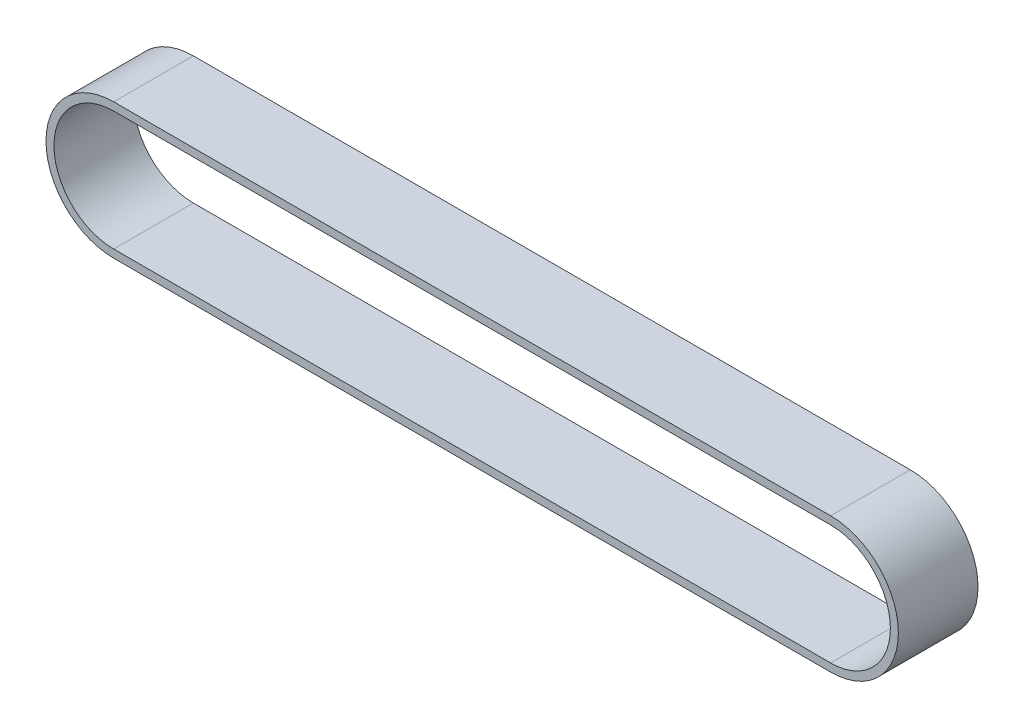
from build123d import *

# Parameters (mm, degrees)
EXTRUDE_1_DEPTH = 50


with BuildPart() as part:
    # 草图1 → 凸台-拉伸1 (new body)
    with BuildSketch(Plane.XY):
        with BuildLine():
            Line((-225, 42.5), (225, 42.5))
            ThreePointArc((225, 42.5), (267.5, 0), (225, -42.5))
            Line((225, -42.5), (-225, -42.5))
            ThreePointArc((-225, -42.5), (-267.5, 0), (-225, 42.5))
        make_face()
        with BuildLine():
            Line((-225, 37.5), (225, 37.5))
            ThreePointArc((225, 37.5), (262.5, 0), (225, -37.5))
            Line((225, -37.5), (-225, -37.5))
            ThreePointArc((-225, -37.5), (-262.5, 0), (-225, 37.5))
        make_face(mode=Mode.SUBTRACT)
    extrude(amount=EXTRUDE_1_DEPTH)


solid = part.part
